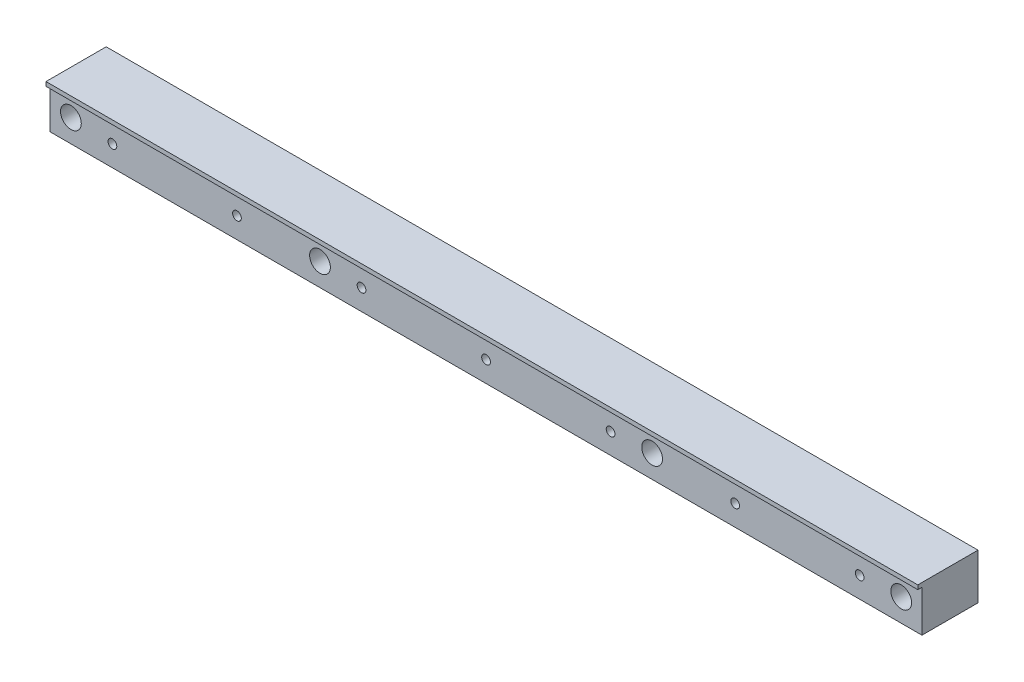
SolidWorks part; units mm, degrees
ref_plane "Front Plane" through (0, 0, 0) normal (0, 0, 1) x (1, 0, 0)
ref_plane "Top Plane" through (0, 0, 0) normal (0, 1, 0) x (1, 0, 0)
ref_plane "Right Plane" through (0, 0, 0) normal (1, 0, 0) x (0, 0, -1)
sketch "Sketch1" plane through (0, 0, 0) normal (0, 0, 1) x (1, 0, 0)
  line L1 (-210, -11) -> (210, -11)
  line L2 (-210, -11) -> (-210, 11)
  line L3 (-210, 11) -> (210, 11)
  line L4 (210, -11) -> (210, 11)
  line L5 (-210, -11) -> (210, 11) construction
  line L6 (-210, 11) -> (210, -11) construction
  point P0 (0, 0)
  dimension "D1" = 420
  dimension "D2" = 22
extrude "Boss-Extrude1" add sketch "Sketch1" along normal blind 27
sketch "Sketch2" plane through (0, 0, 27) normal (0, 0, 1) x (1, 0, 0)
  line L0 (210, -11) -> (210, 11) construction
  line L1 (-210, 11) -> (210, 11)
  line L2 (-210, 11) -> (-210, 9)
  line L3 (-210, 9) -> (210, 9)
  line L4 (210, 11) -> (210, 9)
  dimension "D1" = 2
extrude "Boss-Extrude2" add sketch "Sketch2" along normal blind 2
hole_wizard "M5 Tapped Hole1" positions "Sketch5" profile "Sketch6" tap size "M5" standard "ISO"
sketch "Sketch5" plane through (0, 0, 27) normal (0, 0, 1) x (1, 0, 0)
  point P0 (180, -1)
  point P3 (120, -1)
  point P6 (60, -1)
  point P9 (0, -1)
  point P12 (-180, -1)
  point P15 (-120, -1)
  point P18 (-60, -1)
sketch "Sketch6" plane through (180, -1, 27) normal (1, 0, 0) x (0, -1, 0)
  line L0 (0, 0) -> (0, 13.6618)
  line L1 (0, 13.6618) -> (2.1, 12.4)
  line L2 (2.1, 12.4) -> (2.1, 0)
  line L5 (2.1, 0) -> (0, 0)
  line L10 (0, 13.6618) -> (-2.1, 12.4) construction
  line L11 (0, -6.35) -> (0, 107.95) construction
  dimension "螺纹孔钻头直径" = 4.2
  dimension "螺纹孔钻头深度" = 12.4
  dimension "导头角度" = 118
cosmetic thread "Cosmetic Thread1"
cosmetic thread "Cosmetic Thread2"
cosmetic thread "Cosmetic Thread3"
cosmetic thread "Cosmetic Thread4"
cosmetic thread "Cosmetic Thread5"
cosmetic thread "Cosmetic Thread6"
cosmetic thread "Cosmetic Thread7"
hole_wizard "CBORE for M5 Hex Socket Head Cap Screw1" positions "Sketch7" profile "Sketch8" counterbore size "M5" standard "ISO" end condition through all
sketch "Sketch7" plane through (0, 0, 27) normal (0, 0, 1) x (1, 0, 0)
  line L0 (200, 0) -> (80, 0) construction
  line L1 (80, 0) -> (0, 0) construction
  line L2 (0, 0) -> (0, 66.1887) construction
  point P0 (200, 0)
  point P2 (80, 0)
  point P13 (-80, 0)
  point P14 (-200, 0)
  dimension "D1" = 160
  dimension "D2" = 120
sketch "Sketch8" plane through (200, 0, 27) normal (1, 0, 0) x (0, -1, 0)
  line L0 (0, 0) -> (0, 27)
  line L1 (0, 27) -> (2.75, 27)
  line L3 (2.75, 27) -> (2.75, 17)
  line L4 (2.75, 17) -> (5, 17)
  line L5 (5, 17) -> (5, 0)
  line L7 (5, 0) -> (0, 0)
  line L11 (0, -6.35) -> (0, 107.95) construction
  dimension "通孔孔直径" = 5.5
  dimension "通孔孔深度" = 27
  dimension "柱形沉头孔直径" = 10
  dimension "柱形沉头孔深度" = 17
